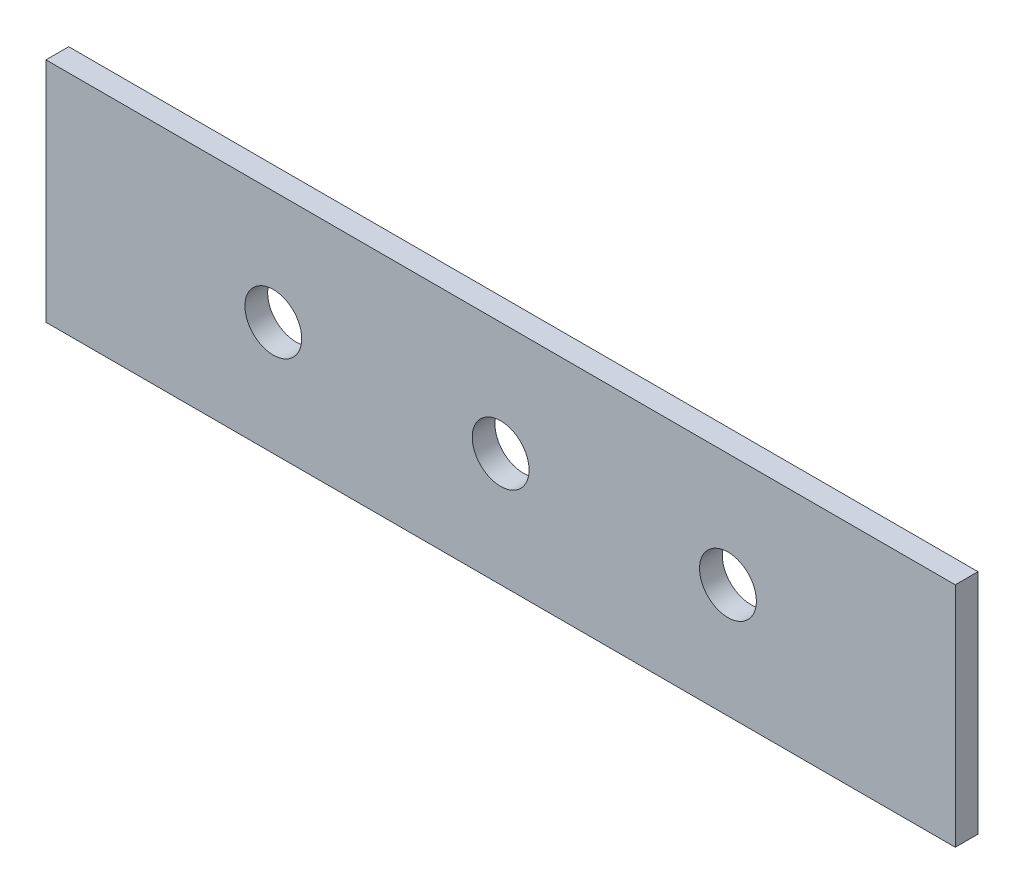
SolidWorks part; units mm, degrees
ref_plane "前视基准面" through (0, 0, 0) normal (0, 0, 1) x (1, 0, 0)
ref_plane "上视基准面" through (0, 0, 0) normal (0, 1, 0) x (1, 0, 0)
ref_plane "右视基准面" through (0, 0, 0) normal (1, 0, 0) x (0, 0, -1)
sketch "草图1" plane through (0, 0, 0) normal (0, 0, 1) x (1, 0, 0)
  line L0 (0, 0) -> (0, 80)
  line L1 (0, 80) -> (310, 80)
  line L2 (310, 80) -> (320, 80)
  line L3 (320, 80) -> (320, 0)
  line L4 (320, 0) -> (0, 0)
extrude "凸台-拉伸1" add sketch "草图1" along normal blind 8
sketch "草图2" plane through (0, 0, 8) normal (0, 0, 1) x (1, 0, 0)
  line L0 (0, 40) -> (80, 40)
  line L1 (0, 80) -> (0, 0) construction
  line L2 (80, 40) -> (160, 40)
  line L3 (160, 40) -> (240, 40)
  circle A0 centre (80, 40) radius 10
  circle A1 centre (160, 40) radius 10
  circle A2 centre (240, 40) radius 10
extrude "切除-拉伸1" cut sketch "草图2" against normal blind 24
